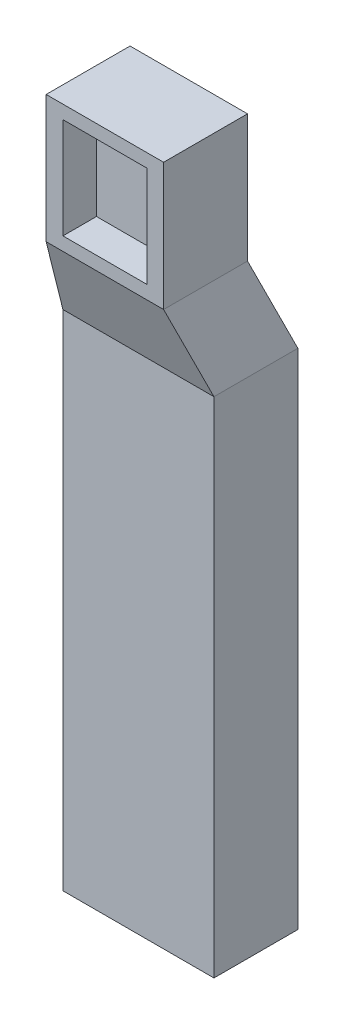
from build123d import *

# Parameters (mm, degrees)
BOSS_EXTRUDE1_DEPTH = 350
CUT_EXTRUDE1_DEPTH  = 2023.028684267
SKETCH4_W           = 250
SKETCH4_H           = 300
CUT_EXTRUDE2_DEPTH  = 100


with BuildPart() as part:
    # Sketch2 → Boss-Extrude1 (new body)
    with BuildSketch(Plane.XY):
        Polygon((-175, 190), (175, 190), (175, -190), (225, -440), (225, -1940), (-225, -1940), (-225, -440), (-175, -190), align=None)
    extrude(amount=BOSS_EXTRUDE1_DEPTH)

    # Sketch3 → Cut-Extrude1 (cut, through all)
    with BuildSketch(Plane.ZY.offset(225)):
        Polygon((350, -190), (250, -440), (250, -1940), (350, -1940), align=None)
        Polygon((0, -440), (100, -190), (100, 190), (0, 190), align=None)
    extrude(amount=-CUT_EXTRUDE1_DEPTH, mode=Mode.SUBTRACT)

    # Sketch4 → Cut-Extrude2 (cut)
    with BuildSketch(Plane.XY.offset(350)):
        Rectangle(SKETCH4_W, SKETCH4_H)
    extrude(amount=-CUT_EXTRUDE2_DEPTH, mode=Mode.SUBTRACT)


solid = part.part
